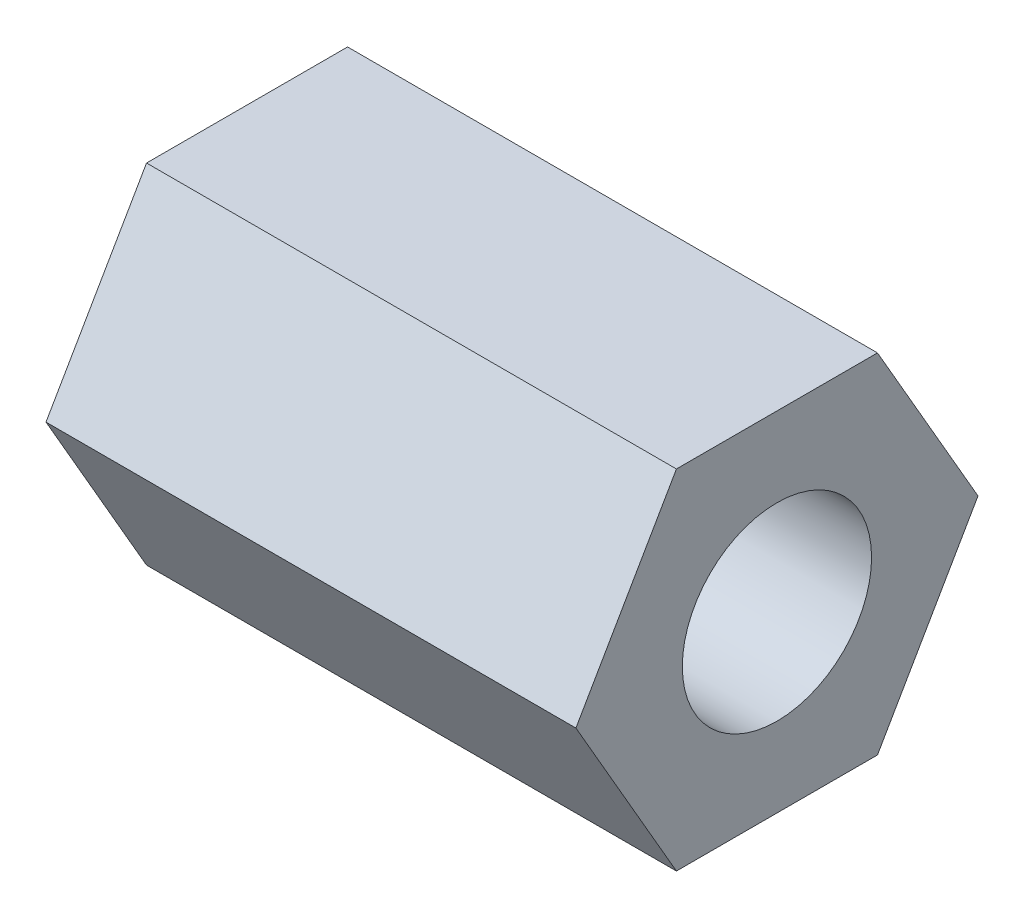
SolidWorks part; units mm, degrees
material "黄铜"
ref_plane "前视基准面" through (0, 0, 0) normal (0, 0, 1) x (1, 0, 0)
ref_plane "上视基准面" through (0, 0, 0) normal (0, 1, 0) x (1, 0, 0)
ref_plane "右视基准面" through (0, 0, 0) normal (1, 0, 0) x (0, 0, -1)
other "Configuration Table"
sketch "草图1" plane through (0, 0, 0) normal (1, 0, 0) x (0, 0, -1)
  line L1 (2.6558, 0) -> (1.3279, 2.3)
  line L2 (1.3279, 2.3) -> (-1.3279, 2.3)
  line L3 (-1.3279, 2.3) -> (-2.6558, 0)
  line L4 (-2.6558, 0) -> (-1.3279, -2.3)
  line L5 (-1.3279, -2.3) -> (1.3279, -2.3)
  line L6 (1.3279, -2.3) -> (2.6558, 0)
  circle A0 centre (0, 0) radius 2.3 construction
  dimension "D1" = 4.6
extrude "凸台-拉伸1" add sketch "草图1" along normal blind 7
hole_wizard "M3 螺纹孔1" positions "草图2" profile "草图3" tap size "M3" standard "GB" end condition through all
sketch "草图2" plane through (7, 0, 0) normal (1, 0, 0) x (0, 0, -1)
  point P0 (0, 0)
sketch "草图3" plane through (7, 0, 0) normal (0, 1, 0) x (0, 0, -1)
  line L0 (0, 0) -> (0, 7)
  line L1 (0, 7) -> (1.25, 7)
  line L2 (1.25, 7) -> (1.25, 0)
  line L5 (1.25, 0) -> (0, 0)
  line L11 (0, -6.35) -> (0, 107.95) construction
  dimension "通孔螺纹孔钻头直径" = 2.5
  dimension "通孔螺纹孔钻头深度" = 7
cosmetic thread "孔螺蚊线1"
